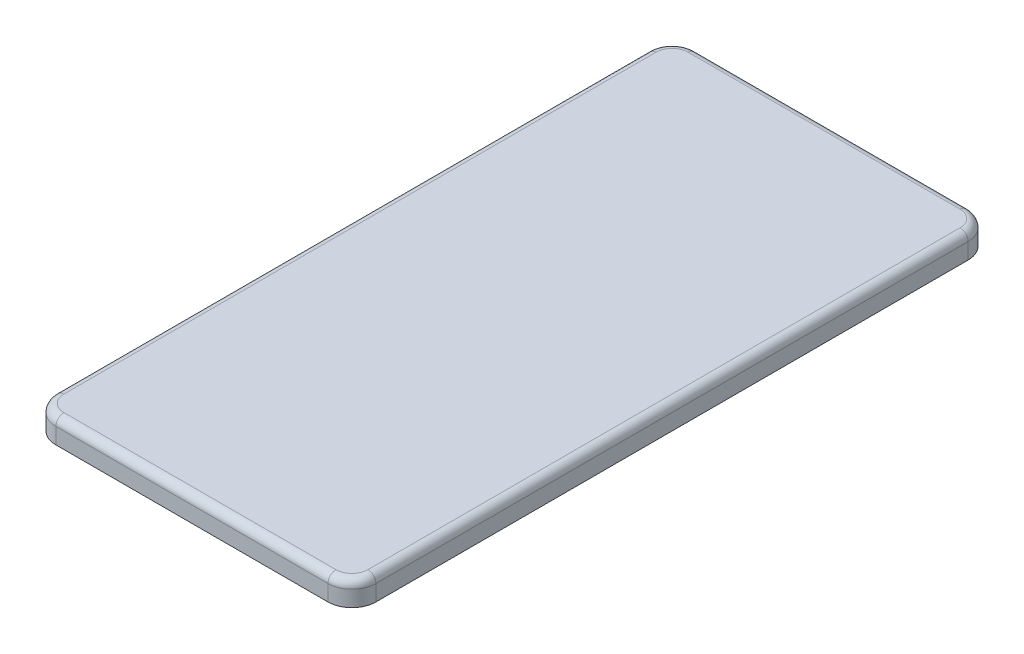
SolidWorks part; units mm, degrees
ref_plane "前视基准面" through (0, 0, 0) normal (0, 0, 1) x (1, 0, 0)
ref_plane "上视基准面" through (0, 0, 0) normal (0, 1, 0) x (1, 0, 0)
ref_plane "右视基准面" through (0, 0, 0) normal (1, 0, 0) x (0, 0, -1)
sketch "草图1" plane through (0, 0, 0) normal (0, 1, 0) x (1, 0, 0)
  line L1 (-20, -40) -> (20, -40)
  line L2 (-20, -40) -> (-20, 40)
  line L3 (-20, 40) -> (20, 40)
  line L4 (20, -40) -> (20, 40)
  line L5 (-20, -40) -> (20, 40) construction
  line L6 (-20, 40) -> (20, -40) construction
  point P0 (0, 0)
  dimension "D1" = 80
  dimension "D2" = 40
extrude "凸台-拉伸1" add sketch "草图1" along normal blind 3
fillet "圆角2" radius 3 4 edges at (-20, 1.5, -40) (20, 1.5, -40) (-20, 1.5, 40) (20, 1.5, 40)
fillet "圆角3" radius 1 8 edges at (19.1213, 3, -39.1213) (20, 3, 0) (19.1213, 3, 39.1213) (0, 3, 40) (-19.1213, 3, 39.1213) (-20, 3, 0) (-19.1213, 3, -39.1213) (0, 3, -40)
